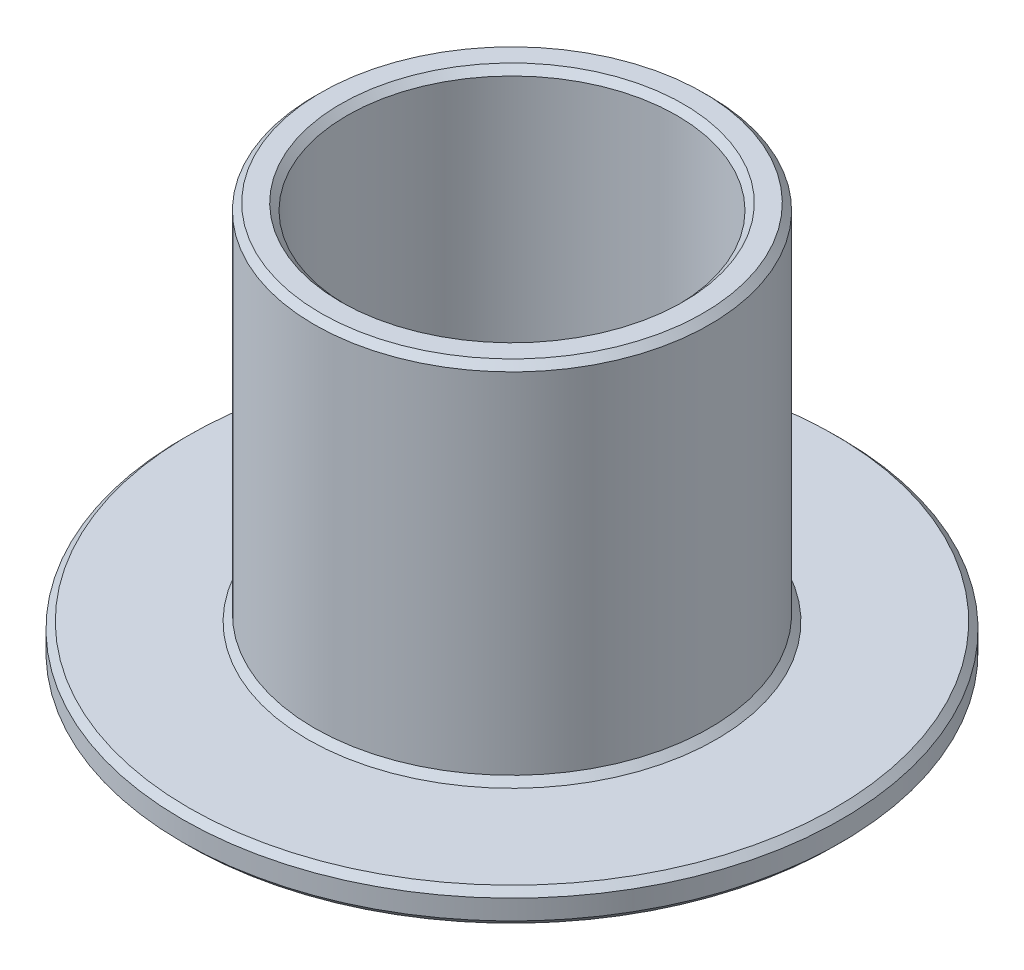
SolidWorks part; units mm, degrees
ref_plane "前视基准面" through (0, 0, 0) normal (0, 0, 1) x (1, 0, 0)
ref_plane "上视基准面" through (0, 0, 0) normal (0, 1, 0) x (1, 0, 0)
ref_plane "右视基准面" through (0, 0, 0) normal (1, 0, 0) x (0, 0, -1)
sketch "草图1" plane through (0, 0, 0) normal (0, 0, 1) x (1, 0, 0)
  line L0 (0, 0) -> (0, 15.0558) construction
  line L1 (2.5, 0) -> (5, 0)
  line L2 (5, 0) -> (5, 0.5)
  line L3 (5, 0.5) -> (3, 0.5)
  line L4 (3, 0.5) -> (3, 6)
  line L5 (3, 6) -> (2.5, 6)
  line L6 (2.5, 6) -> (2.5, 0)
  line L7 (2.5, 0) -> (0, 0) construction
  dimension "D1" = 5
  dimension "D2" = 6
  dimension "D3" = 6
  dimension "D4" = 10
revolve "旋转1" add sketch "草图1" angle 360 about L0
chamfer "倒角1" distance 0.1 angle 45 6 edges at (0, 0, -5) (0, 0.5, -5) (0, 6, -3) (0, 0.5, -3) (0, 0, -2.5) (0, 6, -2.5)
